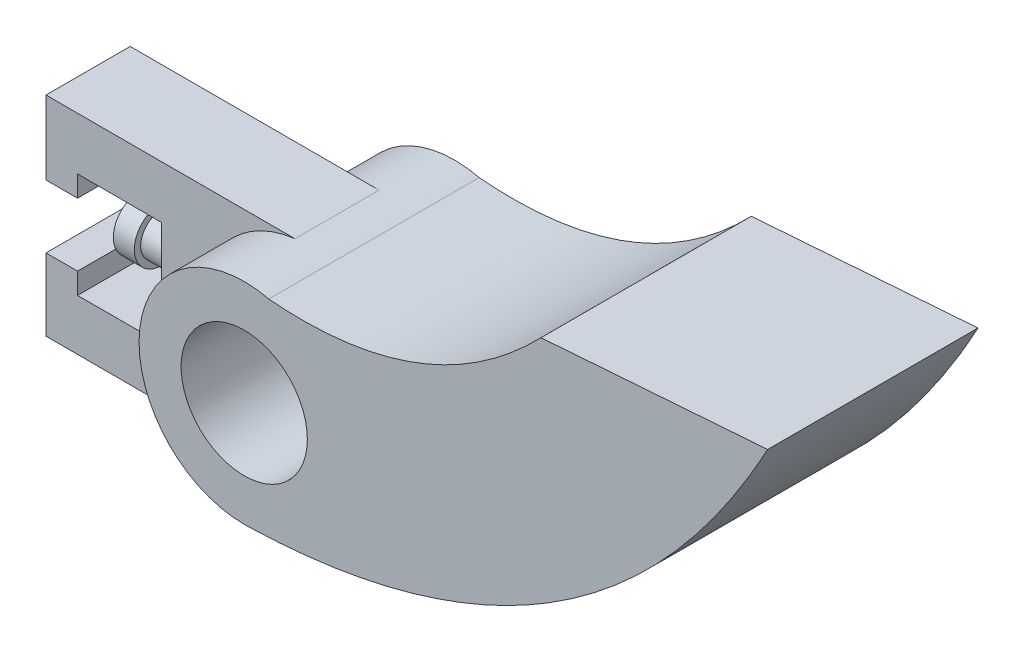
from build123d import *

# Parameters (mm, degrees)
SKETCH1_R           = 5
SKETCH1_R_2         = 3
BOSS_EXTRUDE1_DEPTH = 10
BOSS_EXTRUDE2_START = -10
SKETCH2_R           = 3
BOSS_EXTRUDE2_DEPTH = 10
BOSS_EXTRUDE3_START = -7
BOSS_EXTRUDE3_DEPTH = 4
SKETCH4_W           = 4
SKETCH4_H           = 9.930378158
CUT_EXTRUDE1_DEPTH  = 8
CUT_EXTRUDE3_DEPTH  = 6
SKETCH7_R           = 1
BOSS_EXTRUDE4_DEPTH = 3
SKETCH8_R           = 1.3
BOSS_EXTRUDE5_DEPTH = 1


with BuildPart() as part:
    # Sketch1 → Boss-Extrude1 (new body)
    with BuildSketch(Plane.XY):
        Circle(SKETCH1_R)
        Circle(SKETCH1_R_2, mode=Mode.SUBTRACT)
    extrude(amount=BOSS_EXTRUDE1_DEPTH)

    # Sketch2 → Boss-Extrude2 (add)
    with BuildSketch(Plane.XY.offset(10).offset(BOSS_EXTRUDE2_START)):
        with BuildLine():
            Line((24.88045834, 10.525498272), (14.10478585, 9.738087788))
            add(Edge.make_bspline(
                [(14.10478585, 9.738087788), (8.323441711, 3.769762394), (0, 5)],
                knots=[0, 0, 0, 1, 1, 1], degree=2))
            ThreePointArc((0, 5), (-5, 0), (0, -5))
            add(Edge.make_bspline(
                [(24.88045834, 10.525498272), (16.689881937, -4.631862586), (0, -5)],
                knots=[0, 0, 0, 1, 1, 1], degree=2))
        make_face()
        Circle(SKETCH2_R, mode=Mode.SUBTRACT)
    extrude(amount=BOSS_EXTRUDE2_DEPTH)

    # Sketch3 → Boss-Extrude3 (add)
    with BuildSketch(Plane.XY.offset(10).offset(BOSS_EXTRUDE3_START)):
        with BuildLine():
            Line((-20.423369766, -4.965189079), (0, -4.965189079))
            Line((0, -4.965189079), (0, -3))
            ThreePointArc((0, -3), (-3, 0), (0, 3))
            Line((0, 3), (0, 4.965189079))
            Line((0, 4.965189079), (-20.423369766, 4.965189079))
            Line((-20.423369766, 4.965189079), (-20.423369766, -4.965189079))
        make_face()
    extrude(amount=BOSS_EXTRUDE3_DEPTH)

    # Sketch4 → Cut-Extrude1 (cut)
    with BuildSketch(Plane.ZY.offset(20.423369766)):
        with Locations((5, 0)):
            Rectangle(SKETCH4_W, SKETCH4_H)
    extrude(amount=-CUT_EXTRUDE1_DEPTH, mode=Mode.SUBTRACT)

    # Sketch6 → Cut-Extrude3 (cut)
    with BuildSketch(Plane.XY.offset(7)):
        Polygon((-12.423369766, 1.465189079), (-10.923369766, 1.465189079), (-10.923369766, 2.465189079), (-6.923369766, 2.465189079), (-6.923369766, -2.534810921), (-10.923369766, -2.534810921), (-10.923369766, -1.534810921), (-12.423369766, -1.534810921), align=None)
    extrude(amount=-CUT_EXTRUDE3_DEPTH, mode=Mode.SUBTRACT)

    # Sketch7 → Boss-Extrude4 (add)
    with BuildSketch(Plane.ZY.offset(6.923369766)):
        with Locations(Location((5, 0, 0), (0, 0, 90))):
            Circle(SKETCH7_R)
    extrude(amount=BOSS_EXTRUDE4_DEPTH)

    # Sketch8 → Boss-Extrude5 (add)
    with BuildSketch(Plane.ZY.offset(9.923369766)):
        with Locations(Location((5, 0, 0), (0, 0, 270))):
            Circle(SKETCH8_R)
    extrude(amount=-BOSS_EXTRUDE5_DEPTH)


solid = part.part
